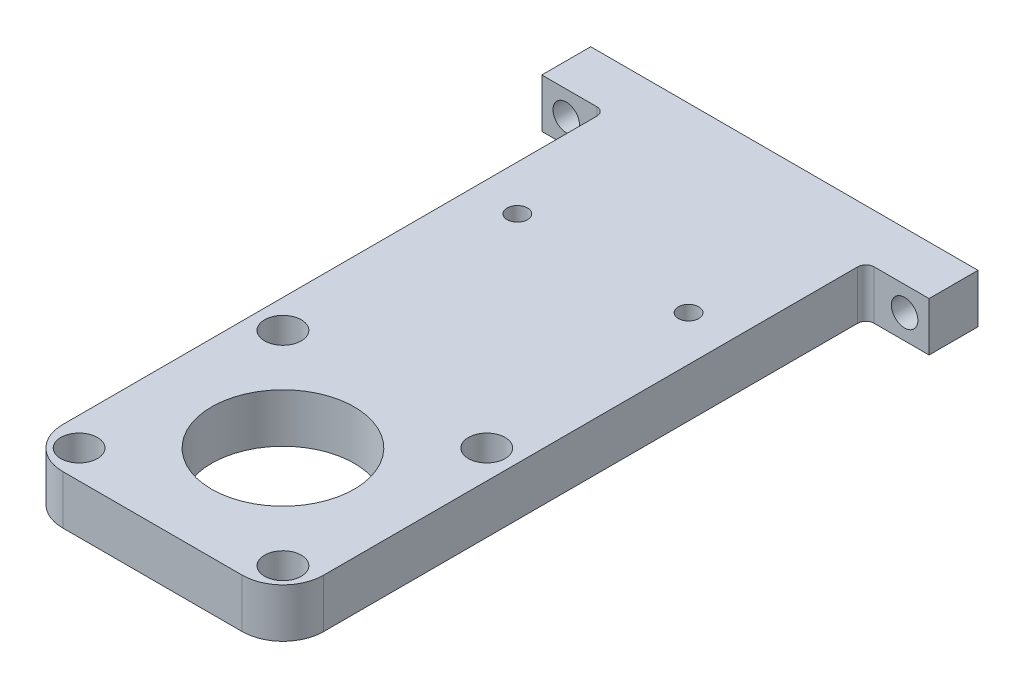
from build123d import *

# Parameters (mm, degrees)
SKETCH_1_W                = 95
SKETCH_1_H                = 155
EXTRUDE_1_DEPTH           = 12
SKETCH_9_W                = 15.5
SKETCH_9_H                = 143
CUT_EXTRUDE_4_DEPTH       = 183.1922062
HOLE_WIZARD_6_5_6_5_1_D   = 6.5
SKETCH_12_R               = 17.5
CUT_EXTRUDE_5_DEPTH       = 183.1922062
FILLET_1_R                = 10
HOLE_WIZARD_5_0_5_1_D     = 5
HOLE_WIZARD_5_0_5_1_DEPTH = 10
HOLE_WIZARD_5_0_5_1_TIP   = 1.502151548
FILLET_2_R                = 2
HOLE_WIZARD_M6_2_D        = 5
MM_1_D                    = 9


with BuildPart() as part:
    # 草图1 → 凸台-拉伸1 (new body)
    with BuildSketch(Plane(origin=(0, 0, 0), x_dir=(1, 0, 0), z_dir=(0, 1, 0))):
        with Locations((47.5, -77.5)):
            Rectangle(SKETCH_1_W, SKETCH_1_H)
    extrude(amount=EXTRUDE_1_DEPTH)

    # 草图9 → 切除-拉伸4 (cut, through all)
    with BuildSketch(Plane(origin=(0, 12, 0), x_dir=(1, 0, 0), z_dir=(0, 1, 0))):
        with Locations((7.75, -83.5)):
            Rectangle(SKETCH_9_W, SKETCH_9_H)
        with Locations((87.25, -83.5)):
            Rectangle(SKETCH_9_W, SKETCH_9_H)
    extrude(amount=-CUT_EXTRUDE_4_DEPTH, mode=Mode.SUBTRACT)

    # Ø6.5 (6.5) 直径孔1 (through all)
    with Locations(Plane.XY.offset(12)):
        with Locations((6, 6), (89, 6)):
            Hole(HOLE_WIZARD_6_5_6_5_1_D / 2)

    # 草图12 → 切除-拉伸5 (cut, through all)
    with BuildSketch(Plane(origin=(0, 12, 0), x_dir=(1, 0, 0), z_dir=(0, 1, 0))):
        with Locations(Location((47.5, -123, 0), (0, 0, 270))):
            Circle(SKETCH_12_R)
    extrude(amount=-CUT_EXTRUDE_5_DEPTH, mode=Mode.SUBTRACT)

    # 圆角1
    fillet_1_edges = [part.edges().sort_by_distance(p)[0] for p in [
        (15.5, 6, 155),
        (79.5, 6, 155),
    ]]
    fillet(fillet_1_edges, radius=FILLET_1_R)

    # Ø5.0 (5) 直径孔1
    with Locations(Plane(origin=(0, 0, 0), x_dir=(-1, 0, 0), z_dir=(0, 0, -1))):
        with Locations((-67.5, 6), (-27.5, 6)):
            Hole(HOLE_WIZARD_5_0_5_1_D / 2, depth=HOLE_WIZARD_5_0_5_1_DEPTH)
            with Locations((0, 0, -(HOLE_WIZARD_5_0_5_1_DEPTH + HOLE_WIZARD_5_0_5_1_TIP / 2))):  # 118° drill point
                Cone(0, HOLE_WIZARD_5_0_5_1_D / 2, HOLE_WIZARD_5_0_5_1_TIP, mode=Mode.SUBTRACT)

    # 圆角2
    fillet_2_edges = [part.edges().sort_by_distance(p)[0] for p in [
        (15.5, 6, 12),
        (79.5, 6, 12),
    ]]
    fillet(fillet_2_edges, radius=FILLET_2_R)

    # M6 螺纹孔2 (through all)
    with Locations(Plane(origin=(0, 0, 0), x_dir=(-1, 0, 0), z_dir=(0, -1, 0))):
        with Locations((-68.5, -44.5), (-26.5, -44.5)):
            Hole(HOLE_WIZARD_M6_2_D / 2)

    # 大小mm 暗销孔1 (through all)
    with Locations(Plane(origin=(0, 0, 0), x_dir=(-1, 0, 0), z_dir=(0, -1, 0))):
        with Locations((-72.5, -98), (-72.5, -148), (-22.5, -148), (-22.5, -98)):
            Hole(MM_1_D / 2)


solid = part.part
